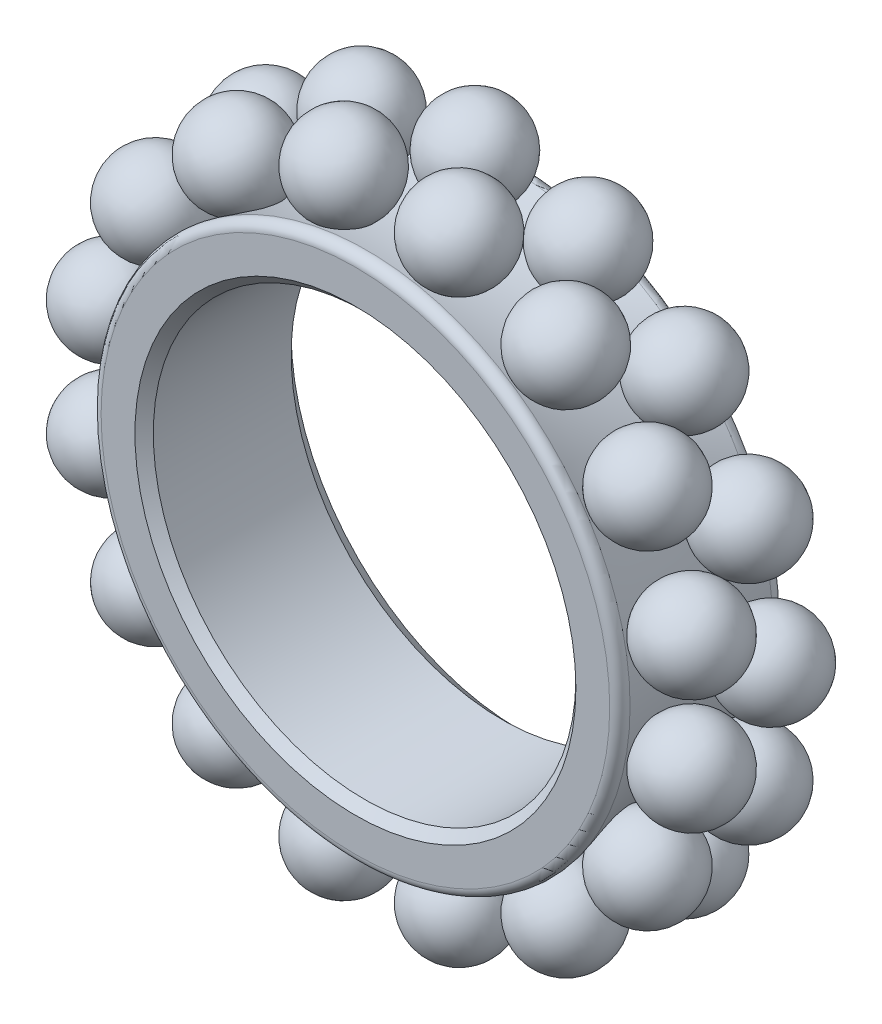
from build123d import *

# Parameters (mm, degrees)
SKETCH1_R           = 29
BOSS_EXTRUDE1_DEPTH = 9
CIRPATTERN4_COUNT   = 16
CIRPATTERN5_COUNT   = 16
SKETCH6_R           = 23
CUT_EXTRUDE1_DEPTH  = 56.614494957
CHAMFER1_SIZE       = 1
CHAMFER2_SIZE       = 2
FILLET1_R           = 1


with BuildPart() as part:
    # Sketch1 → Boss-Extrude1 (new, symmetric)
    with BuildSketch(Plane.XY):
        Circle(SKETCH1_R)
    extrude(amount=BOSS_EXTRUDE1_DEPTH, both=True)

    # Sketch2 → Cut-Revolve1 (revolve, cut)
    with BuildSketch(Plane(origin=(0, 0, 0), x_dir=(1, 0, 0), z_dir=(0, 1, 0))):
        with BuildLine():
            Line((29, 9), (29, -9))
            ThreePointArc((29, -9), (27.664793948, 0), (29, 9))
        make_face()
    revolve(axis=Axis((0, 0, 0), (0, 0, -1)), mode=Mode.SUBTRACT)

    # Sketch6 → Cut-Extrude1 (cut, through all)
    with BuildSketch(Plane.XY.offset(9)):
        Circle(SKETCH6_R)
    extrude(amount=-CUT_EXTRUDE1_DEPTH, mode=Mode.SUBTRACT)

    # Chamfer1
    chamfer1_edges = [part.edges().sort_by_distance(p)[0] for p in [
        (-23, 0, 9),
    ]]
    chamfer(chamfer1_edges, length=CHAMFER1_SIZE)

    # Chamfer2
    chamfer2_edges = [part.edges().sort_by_distance(p)[0] for p in [
        (-23, 0, -9),
    ]]
    chamfer(chamfer2_edges, length=CHAMFER2_SIZE)

    # Fillet1
    fillet1_edges = [part.edges().sort_by_distance(p)[0] for p in [
        (-29, 0, 9),
        (-29, 0, -9),
    ]]
    fillet(fillet1_edges, radius=FILLET1_R)


with BuildPart() as body_2:
    # Sketch3 → Revolve1 (revolve)
    with BuildSketch(Plane(origin=(0, 0, 0), x_dir=(1, 0, 0), z_dir=(0, 1, 0))):
        with BuildLine():
            Line((27.208682114, 4), (37.208682114, 4))
            ThreePointArc((37.208682114, 4), (32.208682114, 9), (27.208682114, 4))
        make_face()
    revolve(axis=Axis((27.208682114, 0, -4), (1, 0, 0)))


with BuildPart() as cirpattern4_1:
    # CirPattern4: pattern copy
    add(body_2.part.rotate(Axis((0, 0, 0), (0, 0, 1)), 1 * 360 / CIRPATTERN4_COUNT))


with BuildPart() as cirpattern4_2:
    # CirPattern4: pattern copy
    add(body_2.part.rotate(Axis((0, 0, 0), (0, 0, 1)), 2 * 360 / CIRPATTERN4_COUNT))


with BuildPart() as cirpattern4_3:
    # CirPattern4: pattern copy
    add(body_2.part.rotate(Axis((0, 0, 0), (0, 0, 1)), 3 * 360 / CIRPATTERN4_COUNT))


with BuildPart() as cirpattern4_4:
    # CirPattern4: pattern copy
    add(body_2.part.rotate(Axis((0, 0, 0), (0, 0, 1)), 4 * 360 / CIRPATTERN4_COUNT))


with BuildPart() as cirpattern4_5:
    # CirPattern4: pattern copy
    add(body_2.part.rotate(Axis((0, 0, 0), (0, 0, 1)), 5 * 360 / CIRPATTERN4_COUNT))


with BuildPart() as cirpattern4_6:
    # CirPattern4: pattern copy
    add(body_2.part.rotate(Axis((0, 0, 0), (0, 0, 1)), 6 * 360 / CIRPATTERN4_COUNT))


with BuildPart() as cirpattern4_7:
    # CirPattern4: pattern copy
    add(body_2.part.rotate(Axis((0, 0, 0), (0, 0, 1)), 7 * 360 / CIRPATTERN4_COUNT))


with BuildPart() as cirpattern4_8:
    # CirPattern4: pattern copy
    add(body_2.part.rotate(Axis((0, 0, 0), (0, 0, 1)), 8 * 360 / CIRPATTERN4_COUNT))


with BuildPart() as cirpattern4_9:
    # CirPattern4: pattern copy
    add(body_2.part.rotate(Axis((0, 0, 0), (0, 0, 1)), 9 * 360 / CIRPATTERN4_COUNT))


with BuildPart() as cirpattern4_10:
    # CirPattern4: pattern copy
    add(body_2.part.rotate(Axis((0, 0, 0), (0, 0, 1)), 10 * 360 / CIRPATTERN4_COUNT))


with BuildPart() as cirpattern4_11:
    # CirPattern4: pattern copy
    add(body_2.part.rotate(Axis((0, 0, 0), (0, 0, 1)), 11 * 360 / CIRPATTERN4_COUNT))


with BuildPart() as cirpattern4_12:
    # CirPattern4: pattern copy
    add(body_2.part.rotate(Axis((0, 0, 0), (0, 0, 1)), 12 * 360 / CIRPATTERN4_COUNT))


with BuildPart() as cirpattern4_13:
    # CirPattern4: pattern copy
    add(body_2.part.rotate(Axis((0, 0, 0), (0, 0, 1)), 13 * 360 / CIRPATTERN4_COUNT))


with BuildPart() as cirpattern4_14:
    # CirPattern4: pattern copy
    add(body_2.part.rotate(Axis((0, 0, 0), (0, 0, 1)), 14 * 360 / CIRPATTERN4_COUNT))


with BuildPart() as cirpattern4_15:
    # CirPattern4: pattern copy
    add(body_2.part.rotate(Axis((0, 0, 0), (0, 0, 1)), 15 * 360 / CIRPATTERN4_COUNT))


with BuildPart() as body_18:
    # Sketch5 → Revolve2 (revolve)
    with BuildSketch(Plane(origin=(0, 0, 0), x_dir=(0.8314696123025446, 0.5555702330196034, 0), z_dir=(-0.5555702330196033, 0.8314696123025445, 0))):
        with BuildLine():
            Line((27.208682114, -4), (37.208682114, -4))
            ThreePointArc((37.208682114, -4), (32.208682114, -9), (27.208682114, -4))
        make_face()
    revolve(axis=Axis((22.623192369, 15.116333862, 4), (0.8314696123025445, 0.5555702330196036, 0)))


with BuildPart() as cirpattern5_1:
    # CirPattern5: pattern copy
    add(body_18.part.rotate(Axis((0, 0, 0), (0, 0, 1)), 1 * 360 / CIRPATTERN5_COUNT))


with BuildPart() as cirpattern5_2:
    # CirPattern5: pattern copy
    add(body_18.part.rotate(Axis((0, 0, 0), (0, 0, 1)), 2 * 360 / CIRPATTERN5_COUNT))


with BuildPart() as cirpattern5_3:
    # CirPattern5: pattern copy
    add(body_18.part.rotate(Axis((0, 0, 0), (0, 0, 1)), 3 * 360 / CIRPATTERN5_COUNT))


with BuildPart() as cirpattern5_4:
    # CirPattern5: pattern copy
    add(body_18.part.rotate(Axis((0, 0, 0), (0, 0, 1)), 4 * 360 / CIRPATTERN5_COUNT))


with BuildPart() as cirpattern5_5:
    # CirPattern5: pattern copy
    add(body_18.part.rotate(Axis((0, 0, 0), (0, 0, 1)), 5 * 360 / CIRPATTERN5_COUNT))


with BuildPart() as cirpattern5_6:
    # CirPattern5: pattern copy
    add(body_18.part.rotate(Axis((0, 0, 0), (0, 0, 1)), 6 * 360 / CIRPATTERN5_COUNT))


with BuildPart() as cirpattern5_7:
    # CirPattern5: pattern copy
    add(body_18.part.rotate(Axis((0, 0, 0), (0, 0, 1)), 7 * 360 / CIRPATTERN5_COUNT))


with BuildPart() as cirpattern5_8:
    # CirPattern5: pattern copy
    add(body_18.part.rotate(Axis((0, 0, 0), (0, 0, 1)), 8 * 360 / CIRPATTERN5_COUNT))


with BuildPart() as cirpattern5_9:
    # CirPattern5: pattern copy
    add(body_18.part.rotate(Axis((0, 0, 0), (0, 0, 1)), 9 * 360 / CIRPATTERN5_COUNT))


with BuildPart() as cirpattern5_10:
    # CirPattern5: pattern copy
    add(body_18.part.rotate(Axis((0, 0, 0), (0, 0, 1)), 10 * 360 / CIRPATTERN5_COUNT))


with BuildPart() as cirpattern5_11:
    # CirPattern5: pattern copy
    add(body_18.part.rotate(Axis((0, 0, 0), (0, 0, 1)), 11 * 360 / CIRPATTERN5_COUNT))


with BuildPart() as cirpattern5_12:
    # CirPattern5: pattern copy
    add(body_18.part.rotate(Axis((0, 0, 0), (0, 0, 1)), 12 * 360 / CIRPATTERN5_COUNT))


with BuildPart() as cirpattern5_13:
    # CirPattern5: pattern copy
    add(body_18.part.rotate(Axis((0, 0, 0), (0, 0, 1)), 13 * 360 / CIRPATTERN5_COUNT))


with BuildPart() as cirpattern5_14:
    # CirPattern5: pattern copy
    add(body_18.part.rotate(Axis((0, 0, 0), (0, 0, 1)), 14 * 360 / CIRPATTERN5_COUNT))


with BuildPart() as cirpattern5_15:
    # CirPattern5: pattern copy
    add(body_18.part.rotate(Axis((0, 0, 0), (0, 0, 1)), 15 * 360 / CIRPATTERN5_COUNT))


solid = Compound([part.part, body_2.part, cirpattern4_1.part, cirpattern4_2.part, cirpattern4_3.part, cirpattern4_4.part, cirpattern4_5.part, cirpattern4_6.part, cirpattern4_7.part, cirpattern4_8.part, cirpattern4_9.part, cirpattern4_10.part, cirpattern4_11.part, cirpattern4_12.part, cirpattern4_13.part, cirpattern4_14.part, cirpattern4_15.part, body_18.part, cirpattern5_1.part, cirpattern5_2.part, cirpattern5_3.part, cirpattern5_4.part, cirpattern5_5.part, cirpattern5_6.part, cirpattern5_7.part, cirpattern5_8.part, cirpattern5_9.part, cirpattern5_10.part, cirpattern5_11.part, cirpattern5_12.part, cirpattern5_13.part, cirpattern5_14.part, cirpattern5_15.part])
